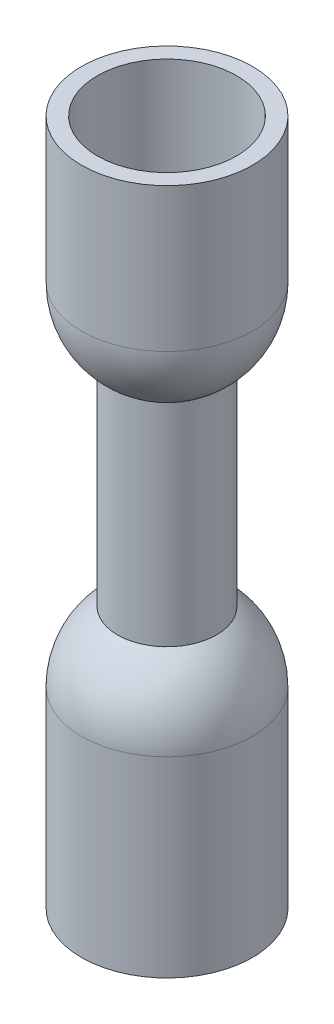
from build123d import *


with BuildPart() as part:
    # Sketch1 → Revolve-Thin1 (revolve)
    with BuildSketch(Plane.XY, mode=Mode.PRIVATE) as revolve_thin1_sk:
        with BuildLine():
            Line((-2.18, 21.493868799), (-2.18, 16.993868799))
            ThreePointArc((-2.18, 16.993868799), (-1.876352845, 15.884048994), (-1.05, 15.083397653))
            Line((-1.05, 15.083397653), (-1.05, 7.910471146))
            ThreePointArc((-1.05, 7.910471146), (-1.876352845, 7.109819805), (-2.18, 6))
            Line((-2.18, 6), (-2.18, 0))
            Line((-2.18, 0), (-2.68, 0))
            Line((-2.68, 0), (-2.68, 6))
            ThreePointArc((-2.68, 6), (-2.380798185, 7.230528342), (-1.55, 8.186298241))
            Line((-1.55, 8.186298241), (-1.55, 14.807570558))
            ThreePointArc((-1.55, 14.807570558), (-2.380798185, 15.763340457), (-2.68, 16.993868799))
            Line((-2.68, 16.993868799), (-2.68, 21.493868799))
            Line((-2.68, 21.493868799), (-2.18, 21.493868799))
        make_face()
    revolve(revolve_thin1_sk.sketch.rotate(Axis((0, 24.17230999, 0), (0, -1, 0)), 270), axis=Axis((0, 24.17230999, 0), (0, -1, 0)))


solid = part.part
